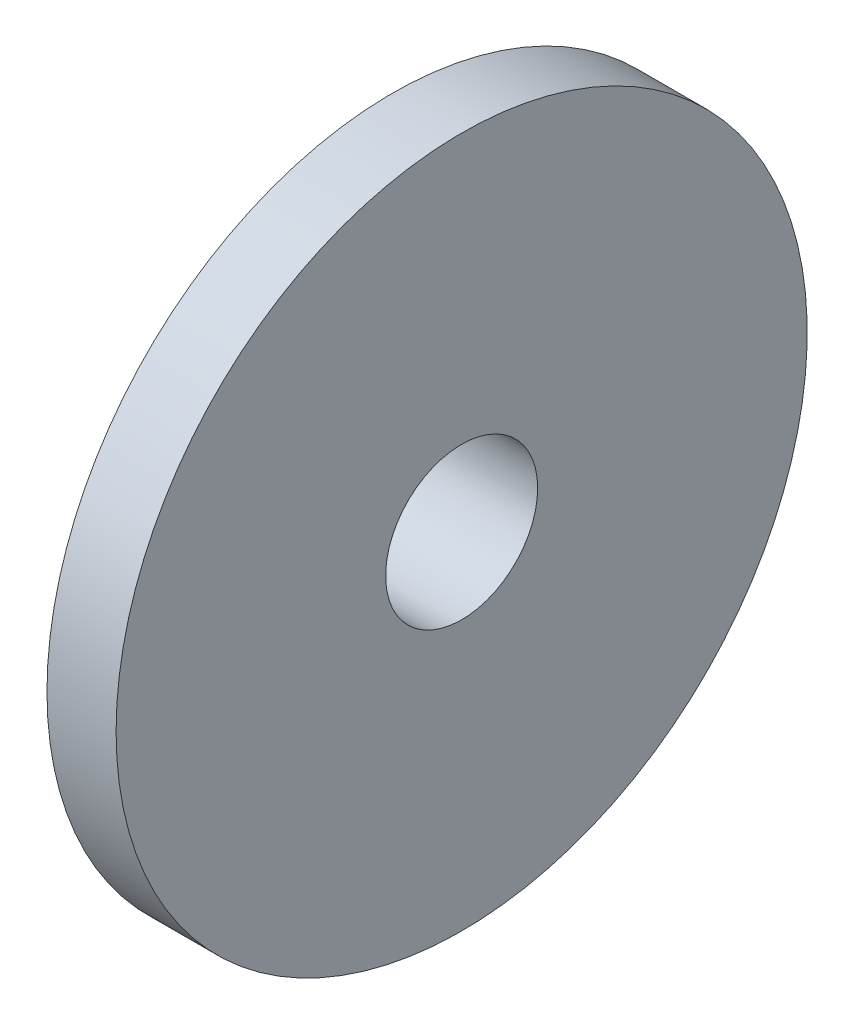
SolidWorks part; units mm, degrees
ref_plane "Front Plane" through (0, 0, 0) normal (0, 0, 1) x (1, 0, 0)
ref_plane "Top Plane" through (0, 0, 0) normal (0, 1, 0) x (1, 0, 0)
ref_plane "Right Plane" through (0, 0, 0) normal (1, 0, 0) x (0, 0, -1)
sketch "Sketch1" plane through (0, 0, 0) normal (0, 0, 1) x (1, 0, 0)
  line L0 (0, 0) -> (12, 0) construction
  line L1 (0, 0) -> (0, 15)
  line L2 (0, 15) -> (7, 15)
  line L3 (7, 15) -> (7, 25)
  line L4 (7, 25) -> (12, 25)
  line L5 (12, 25) -> (12, 0)
  line L6 (0, 0) -> (12, 0)
  dimension "D1" = 12
  dimension "D2" = 5
  dimension "D3" = 15
  dimension "D4" = 25
revolve "Revolve1" add sketch "Sketch1" angle 360 about L0
sketch "Sketch2" plane through (12, 0, 0) normal (1, 0, 0) x (0, 0, -1)
  circle A0 centre (0, 0) radius 5.5
  dimension "D1" = 11
extrude "Cut-Extrude1" cut sketch "Sketch2" against normal blind 17
